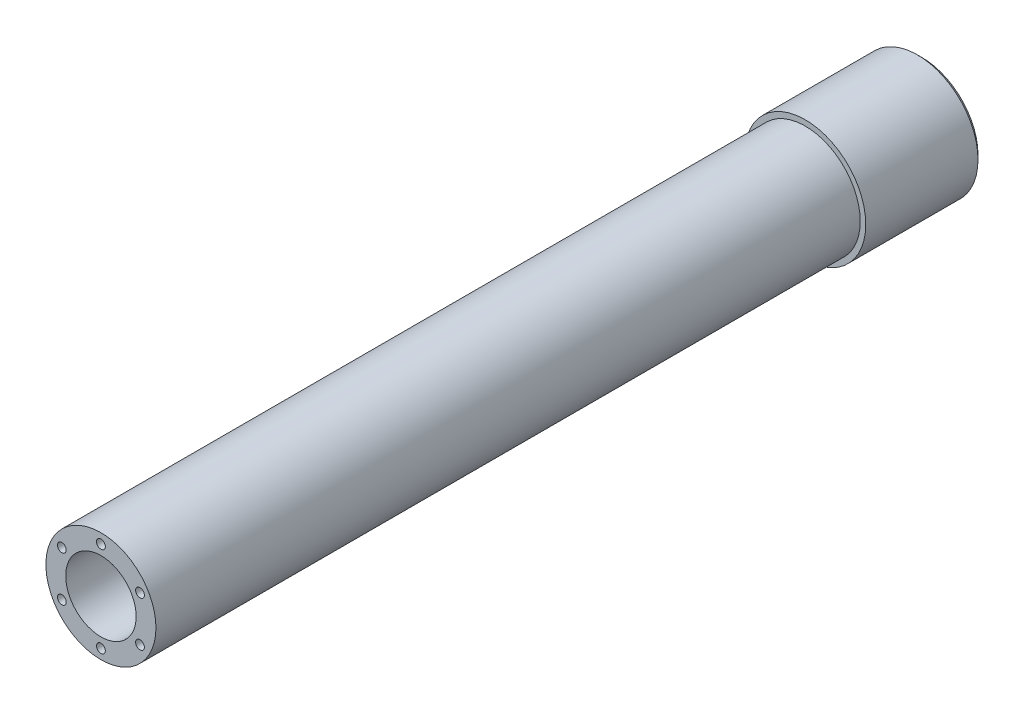
SolidWorks part; units mm, degrees
material "1060 Alloy"
ref_plane "Front Plane" through (0, 0, 0) normal (0, 0, 1) x (1, 0, 0)
ref_plane "Top Plane" through (0, 0, 0) normal (0, 1, 0) x (1, 0, 0)
ref_plane "Right Plane" through (0, 0, 0) normal (1, 0, 0) x (0, 0, -1)
other "Configuration Table"
sketch "Sketch1" plane through (0, 0, 0) normal (0, 0, 1) x (1, 0, 0)
  circle A0 centre (0, 0) radius 16
  circle A1 centre (0, 0) radius 27.5
  dimension "D1" = 32
  dimension "D2" = 55
extrude "Boss-Extrude1" add sketch "Sketch1" along normal blind 53
sketch "Sketch2" plane through (0, 0, 53) normal (0, 0, 1) x (1, 0, 0)
  circle A0 centre (0, 0) radius 16
  circle A1 centre (0, 0) radius 25
  dimension "D1" = 50
extrude "Boss-Extrude2" add sketch "Sketch2" along normal blind 70
sketch "Sketch3" plane through (0, 0, 0) normal (0, 0, -1) x (-1, 0, 0)
  line L0 (0, -38.5559) -> (0, 38.5559) construction
  circle A0 centre (0, 0) radius 19 construction
  circle A2 centre (0, 19) radius 2
  circle A3 centre (13.435, 13.435) radius 2
  circle A4 centre (19, 0) radius 2
  circle A5 centre (13.435, -13.435) radius 2
  circle A6 centre (0, -19) radius 2
  circle A7 centre (-13.435, -13.435) radius 2
  circle A8 centre (-19, 0) radius 2
  circle A9 centre (-13.435, 13.435) radius 2
  point P8 (0, 0)
  point P25 (0, 0)
  dimension "D1" = 38
  dimension "D2" = 4
  dimension "D3" = 8
extrude "Cut-Extrude1" cut sketch "Sketch3" against normal blind 15
chamfer "Chamfer1" distance 2 angle 45 1 edges at (27.5, 0, 0)
sketch "Sketch4" plane through (0, 0, 123) normal (0, 0, 1) x (1, 0, 0)
  circle A0 centre (0, 0) radius 16
  circle A1 centre (0, 0) radius 25
extrude "Boss-Extrude3" add sketch "Sketch4" along normal blind 250
sketch "Sketch5" plane through (0, 0, 373) normal (0, 0, 1) x (1, 0, 0)
  circle A0 centre (0, 0) radius 20.5 construction
  circle A1 centre (0, 20.5) radius 2
  circle A2 centre (17.7535, 10.25) radius 2
  circle A3 centre (17.7535, -10.25) radius 2
  circle A4 centre (0, -20.5) radius 2
  circle A5 centre (-17.7535, -10.25) radius 2
  circle A6 centre (-17.7535, 10.25) radius 2
  point P17 (0, 0)
  dimension "D1" = 41
  dimension "D2" = 4
  dimension "D3" = 6
extrude "Cut-Extrude2" cut sketch "Sketch5" against normal blind 12
